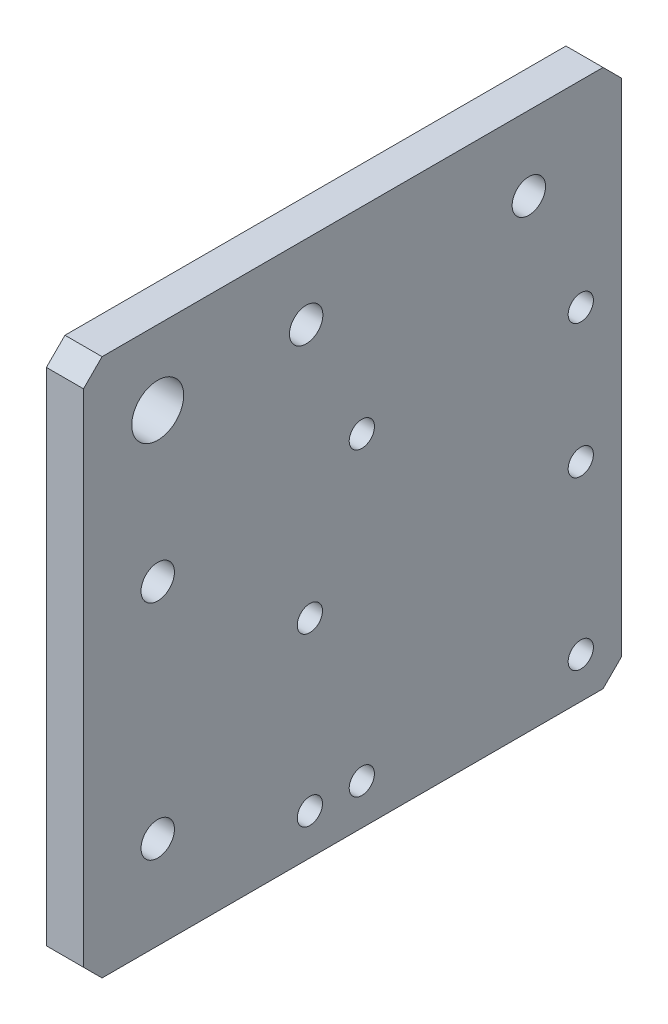
SolidWorks part; units mm, degrees
ref_plane "Front" through (0, 0, 0) normal (0, 0, 1) x (1, 0, 0)
ref_plane "Top" through (0, 0, 0) normal (0, 1, 0) x (1, 0, 0)
ref_plane "Right" through (0, 0, 0) normal (1, 0, 0) x (0, 0, -1)
sketch "草图1" plane through (0, 0, 0) normal (1, 0, 0) x (0, 0, -1)
  line L1 (-72.5, -72.5) -> (72.5, -72.5)
  line L2 (-72.5, -72.5) -> (-72.5, 72.5)
  line L3 (-72.5, 72.5) -> (72.5, 72.5)
  line L4 (72.5, -72.5) -> (72.5, 72.5)
  line L5 (-72.5, -72.5) -> (72.5, 72.5) construction
  line L6 (-72.5, 72.5) -> (72.5, -72.5) construction
  point P0 (0, 0)
  dimension "D1" = 145
  dimension "D2" = 145
extrude "凸台-拉伸1" add sketch "草图1" along normal blind 10
chamfer "倒角1" distance 5 angle 45 4 edges at (5, 72.5, 72.5) (5, 72.5, -72.5) (5, -72.5, -72.5) (5, -72.5, 72.5)
hole_wizard "M8 螺纹孔1" positions "草图4" profile "草图2" tap size "M8" standard "Gb" end condition through all
sketch "草图4" plane through (10, 0, 0) normal (1, 0, 0) x (0, 0, -1)
  line L1 (61.5, -61.5) -> (2.5, -61.5) construction
  line L2 (61.5, -61.5) -> (61.5, 19.5) construction
  line L3 (61.5, 19.5) -> (2.5, 19.5) construction
  line L4 (2.5, -61.5) -> (2.5, 19.5) construction
  line L5 (72.5, -67.5) -> (72.5, 67.5) construction
  line L6 (-67.5, -72.5) -> (67.5, -72.5) construction
  point P0 (61.5, -61.5)
  point P4 (2.5, 19.5)
  point P7 (61.5, 19.5)
  point P8 (2.5, -61.5)
  point P194 (-11.5, -61.5)
  point P196 (-11.5, -16.5)
  point P198 (61.5, -16.5)
  dimension "D1" = 59
  dimension "D2" = 81
  dimension "D3" = 11
  dimension "D4" = 11
  dimension "D5" = 45
  dimension "D6" = 73
cosmetic thread "孔螺蚊线1" parameters "D2"=8
cosmetic thread "孔螺蚊线2" parameters "D2"=8
cosmetic thread "孔螺蚊线3" parameters "D2"=8
cosmetic thread "孔螺蚊线4" parameters "D2"=8
cosmetic thread "孔螺蚊线6" parameters "D2"=8
cosmetic thread "孔螺蚊线7" parameters "D2"=8
cosmetic thread "孔螺蚊线8" parameters "D2"=8
sketch "草图2" plane through (10, -61.5, -61.5) normal (0, 1, 0) x (0, 0, -1)
  line L0 (0, 0) -> (0, 10)
  line L1 (0, 10) -> (3.4, 10)
  line L2 (3.4, 10) -> (3.4, 0)
  line L5 (3.4, 0) -> (0, 0)
  line L11 (0, -6.35) -> (0, 107.95) construction
  dimension "通孔螺纹孔钻头直径" = 6.8
  dimension "通孔螺纹孔钻头深度" = 10
hole_wizard "M16 螺纹孔1" positions "草图7" profile "草图6" tap size "M16" standard "Gb" end condition through all
sketch "草图7" plane through (10, 0, 0) normal (1, 0, 0) x (0, 0, -1)
  line L0 (-72.5, 67.5) -> (-72.5, -67.5) construction
  line L2 (67.5, 72.5) -> (-67.5, 72.5) construction
  point P0 (-52.5, 52.5)
  dimension "D1" = 20
  dimension "D2" = 20
sketch "草图6" plane through (10, 52.5, 52.5) normal (0, 1, 0) x (0, 0, -1)
  line L0 (0, 0) -> (0, 10)
  line L1 (0, 10) -> (7, 10)
  line L2 (7, 10) -> (7, 0)
  line L5 (7, 0) -> (0, 0)
  line L11 (0, -6.35) -> (0, 107.95) construction
  dimension "通孔螺纹孔钻头直径" = 14
  dimension "通孔螺纹孔钻头深度" = 10
cosmetic thread "孔螺蚊线5" parameters "D2"=16
sketch "草图8" plane through (10, 0, 0) normal (1, 0, 0) x (0, 0, -1)
  line L0 (-72.5, 67.5) -> (-72.5, -67.5) construction
  line L1 (-12.5, 52.5) -> (47.5, 52.5) construction
  line L2 (-52.5, 12.5) -> (-52.5, -47.5) construction
  line L3 (67.5, 72.5) -> (-67.5, 72.5) construction
  circle A0 centre (-12.5, 52.5) radius 4.5
  circle A1 centre (47.5, 52.5) radius 4.5
  circle A2 centre (-52.5, 12.5) radius 4.5
  circle A3 centre (-52.5, -47.5) radius 4.5
  dimension "D1" = 9
  dimension "D4" = 60
  dimension "D6" = 20
  dimension "D7" = 20
  dimension "D2" = 60
  dimension "D3" = 60
  dimension "D5" = 60
extrude "切除-拉伸1" cut sketch "草图8" against normal through all
sketch "草图9" plane through (10, 0, 0) normal (1, 0, 0) x (0, 0, -1)
  circle A0 centre (-12.5, 52.5) radius 5.5
  circle A1 centre (47.5, 52.5) radius 5.5
  circle A2 centre (-52.5, 12.5) radius 5.5
  circle A3 centre (-52.5, -47.5) radius 5.5
  dimension "D1" = 11
extrude "切除-拉伸2" [suppressed] cut sketch "草图9" against normal blind 6
